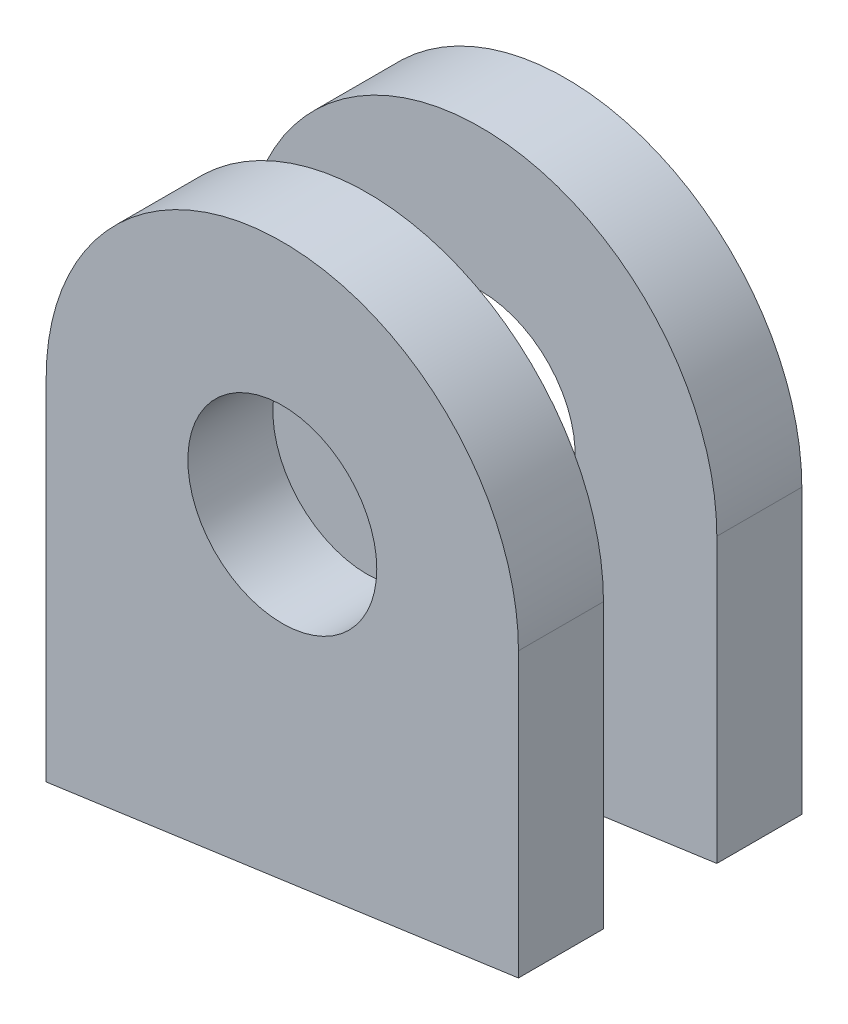
from build123d import *

# Parameters (mm, degrees)
SKETCH1_R               = 12.5
SKETCH1_R_2             = 5
BOSS_EXTRUDE1_DEPTH     = 15
CUT_EXTRUDE1_DEPTH      = 35.536219465
CUT_EXTRUDE1_DEPTH_BACK = 35.536219465
SKETCH2_W               = 6
SKETCH2_H               = 114.982821704


with BuildPart() as part:
    # Sketch1 → Boss-Extrude1 (new body)
    # profile 1 of 2: a face of its own
    with BuildSketch(Plane.XY):
        Circle(SKETCH1_R)
        Circle(SKETCH1_R_2, mode=Mode.SUBTRACT)
    # profile 2 of 2: a face of its own
    with BuildSketch(Plane.XY):
        with BuildLine():
            ThreePointArc((12.5, 0), (0, -12.5), (-12.5, 0))
            Line((-12.5, 0), (-12.5, -18.513520868))
            Line((-12.5, -18.513520868), (12.5, -15))
            Line((12.5, -15), (12.5, 0))
        make_face()
    extrude(amount=BOSS_EXTRUDE1_DEPTH)

    # Sketch2 → Cut-Extrude1 (cut, two sides: drawn at the far end of the back side and taken through both)
    with BuildSketch(Plane(origin=(12.5, 0, 0), x_dir=(0, 0, -1), z_dir=(1, 0, 0)).offset(-CUT_EXTRUDE1_DEPTH_BACK)):
        with Locations((-7.5, 0)):
            Rectangle(SKETCH2_W, SKETCH2_H)
    extrude(amount=CUT_EXTRUDE1_DEPTH + CUT_EXTRUDE1_DEPTH_BACK, mode=Mode.SUBTRACT)


with BuildPart() as cut_extrude1_piece_1:
    # of the separate pieces the step leaves, piece 1, a body of its own (cut_extrude1_pieces)
    add(part.part.solids().sort_by_distance((-12.5, 0, 10.5))[0])


with BuildPart() as cut_extrude1_piece_2:
    # of the separate pieces the step leaves, piece 2, a body of its own (cut_extrude1_pieces)
    add(part.part.solids().sort_by_distance((12.5, 0, 0))[0])


solid = Compound([cut_extrude1_piece_1.part, cut_extrude1_piece_2.part])
